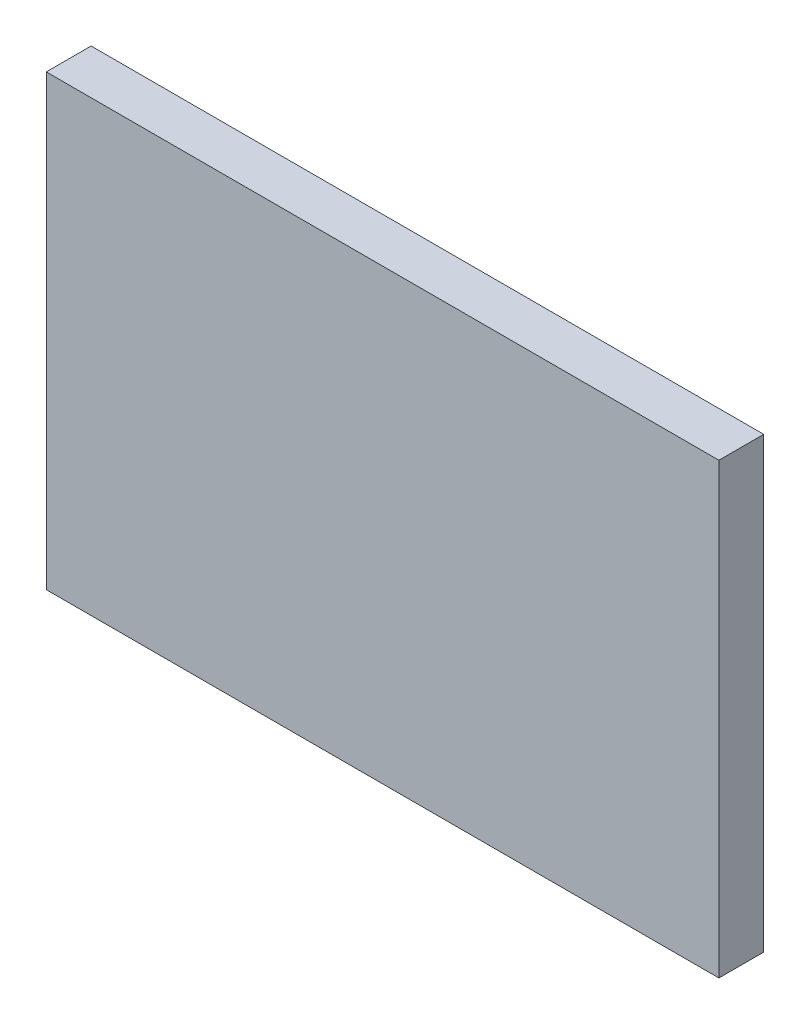
SolidWorks part; units mm, degrees
ref_plane "Front Plane" through (0, 0, 0) normal (0, 0, 1) x (1, 0, 0)
ref_plane "Top Plane" through (0, 0, 0) normal (0, 1, 0) x (1, 0, 0)
ref_plane "Right Plane" through (0, 0, 0) normal (1, 0, 0) x (0, 0, -1)
sketch "Sketch1" plane through (0, 0, 0) normal (0, 0, 1) x (1, 0, 0)
  line L5 (-150, 100) -> (150, 100)
  line L6 (-150, 100) -> (-150, -100)
  line L7 (-150, -100) -> (150, -100)
  line L8 (150, 100) -> (150, -100)
  line L9 (0, -100) -> (0, 100) construction
  line L10 (-150, 0) -> (150, 0) construction
  point P0 (0, 0)
  dimension "D1" = 200
  dimension "D2" = 300
extrude "Boss-Extrude1" add sketch "Sketch1" along normal blind 20
sketch "Sketch2" plane through (0, 0, 0) normal (0, 0, -1) x (-1, 0, 0)
  line L0 (0, 100) -> (0, -102.7637) construction
  line L1 (-150, 100) -> (150, 100) construction
  line L2 (-150, 0) -> (150, 0) construction
  line L3 (-150, -100) -> (-150, 100) construction
  line L4 (150, 100) -> (150, -100) construction
  line L6 (-135, 80) -> (135, 80)
  line L7 (-135, 80) -> (-135, -80)
  line L8 (-135, -80) -> (135, -80)
  line L9 (135, 80) -> (135, -80)
  line L10 (0, -80) -> (0, 80) construction
  line L11 (-135, 0) -> (135, 0) construction
  point P11 (0, 0)
  dimension "D1" = 20
  dimension "D2" = 15
extrude "Cut-Extrude1" cut sketch "Sketch2" against normal blind 10
sketch "Sketch3" plane through (0, 0, 10) normal (0, 0, -1) x (-1, 0, 0)
  line L0 (0, 80) -> (0, -80) construction
  line L2 (135, 80) -> (-135, 80) construction
  line L3 (-135, -80) -> (135, -80) construction
  circle A0 centre (0, 0) radius 30
  dimension "D1" = 60
extrude "Cut-Extrude2" cut sketch "Sketch3" against normal blind 6
